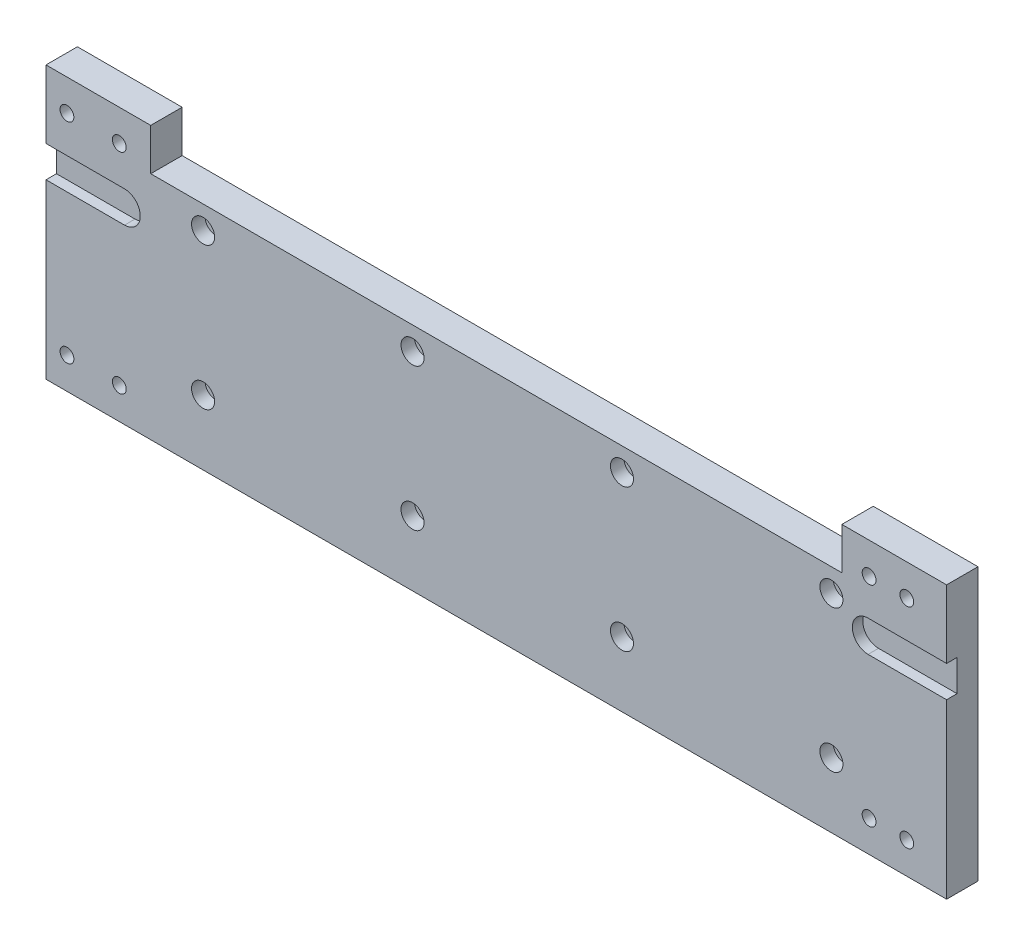
from build123d import *

# Parameters (mm, degrees)
SKETCH1_W                                            = 430
SKETCH1_H                                            = 130
BOSS_EXTRUDE1_DEPTH                                  = 15
HOLE_SIZE_PER_SOCKET_HEAD_CAP_SCREW_TYPE_D           = 6.6
HOLE_SIZE_PER_SOCKET_HEAD_CAP_SCREW_TYPE_CBORE_D     = 11
HOLE_SIZE_PER_SOCKET_HEAD_CAP_SCREW_TYPE_CBORE_DEPTH = 6.8
CUT_EXTRUDE1_DEPTH                                   = 5
CBORE_FOR_M6_HEX_SOCKET_HEAD_CAP_SCREW1_D            = 6.6
CBORE_FOR_M6_HEX_SOCKET_HEAD_CAP_SCREW1_CBORE_D      = 11
CBORE_FOR_M6_HEX_SOCKET_HEAD_CAP_SCREW1_CBORE_DEPTH  = 6.4
SKETCH8_W                                            = 330
SKETCH8_H                                            = 15
CUT_EXTRUDE2_DEPTH                                   = 20


with BuildPart() as part:
    # Sketch1 → Boss-Extrude1 (new body)
    with BuildSketch(Plane.XY):
        with Locations((215, 65)):
            Rectangle(SKETCH1_W, SKETCH1_H)
    extrude(amount=BOSS_EXTRUDE1_DEPTH)

    # Hole size per socket head cap screw type 0 (through all)
    with Locations(Plane(origin=(0, 0, 0), x_dir=(-1, 0, 0), z_dir=(0, 0, -1))):
        with Locations((-10, 15), (-10, 115), (-35, 15), (-35, 115), (-393, 15), (-411, 15), (-393, 115), (-411, 115)):
            CounterBoreHole(HOLE_SIZE_PER_SOCKET_HEAD_CAP_SCREW_TYPE_D / 2, HOLE_SIZE_PER_SOCKET_HEAD_CAP_SCREW_TYPE_CBORE_D / 2, HOLE_SIZE_PER_SOCKET_HEAD_CAP_SCREW_TYPE_CBORE_DEPTH)

    # Sketch5 → Cut-Extrude1 (cut)
    with BuildSketch(Plane.XY.offset(15)):
        with BuildLine():
            Line((430, 97.5), (430, 82.5))
            Line((430, 82.5), (392.5, 82.5))
            ThreePointArc((392.5, 82.5), (385, 90), (392.5, 97.5))
            Line((392.5, 97.5), (430, 97.5))
        make_face()
        with BuildLine():
            Line((37.5, 82.5), (0, 82.5))
            Line((0, 82.5), (0, 97.5))
            Line((0, 97.5), (37.5, 97.5))
            ThreePointArc((37.5, 97.5), (45, 90), (37.5, 82.5))
        make_face()
    extrude(amount=-CUT_EXTRUDE1_DEPTH, mode=Mode.SUBTRACT)

    # CBORE for M6 Hex Socket Head Cap Screw1 (through all)
    with Locations(Plane.XY.offset(15)):
        with Locations((75, 99), (175, 99), (75, 31), (175, 31), (275, 99), (275, 31), (375, 99), (375, 31)):
            CounterBoreHole(CBORE_FOR_M6_HEX_SOCKET_HEAD_CAP_SCREW1_D / 2, CBORE_FOR_M6_HEX_SOCKET_HEAD_CAP_SCREW1_CBORE_D / 2, CBORE_FOR_M6_HEX_SOCKET_HEAD_CAP_SCREW1_CBORE_DEPTH)

    # Sketch8 → Cut-Extrude2 (cut)
    with BuildSketch(Plane(origin=(0, 130, 0), x_dir=(1, 0, 0), z_dir=(0, 1, 0))):
        with Locations((215, -7.5)):
            Rectangle(SKETCH8_W, SKETCH8_H)
    extrude(amount=-CUT_EXTRUDE2_DEPTH, mode=Mode.SUBTRACT)


solid = part.part
